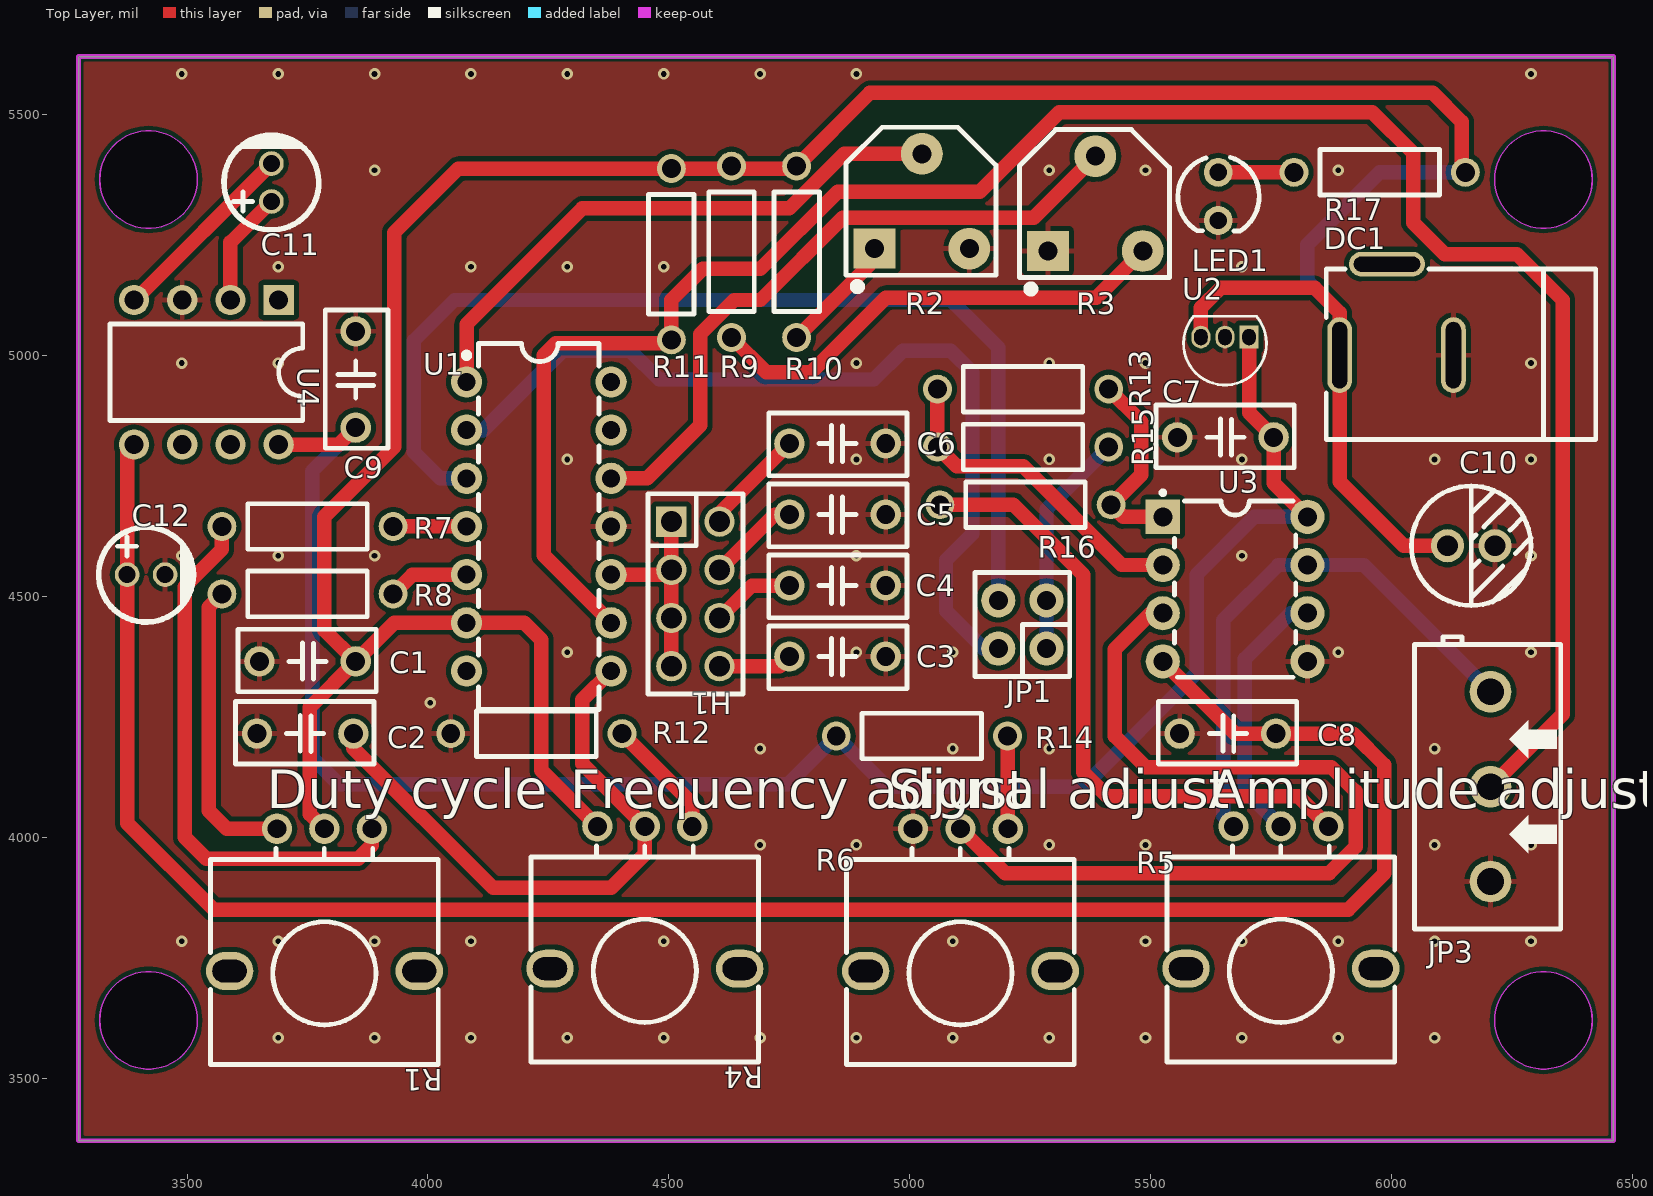
[diagram p0: Top Layer view]
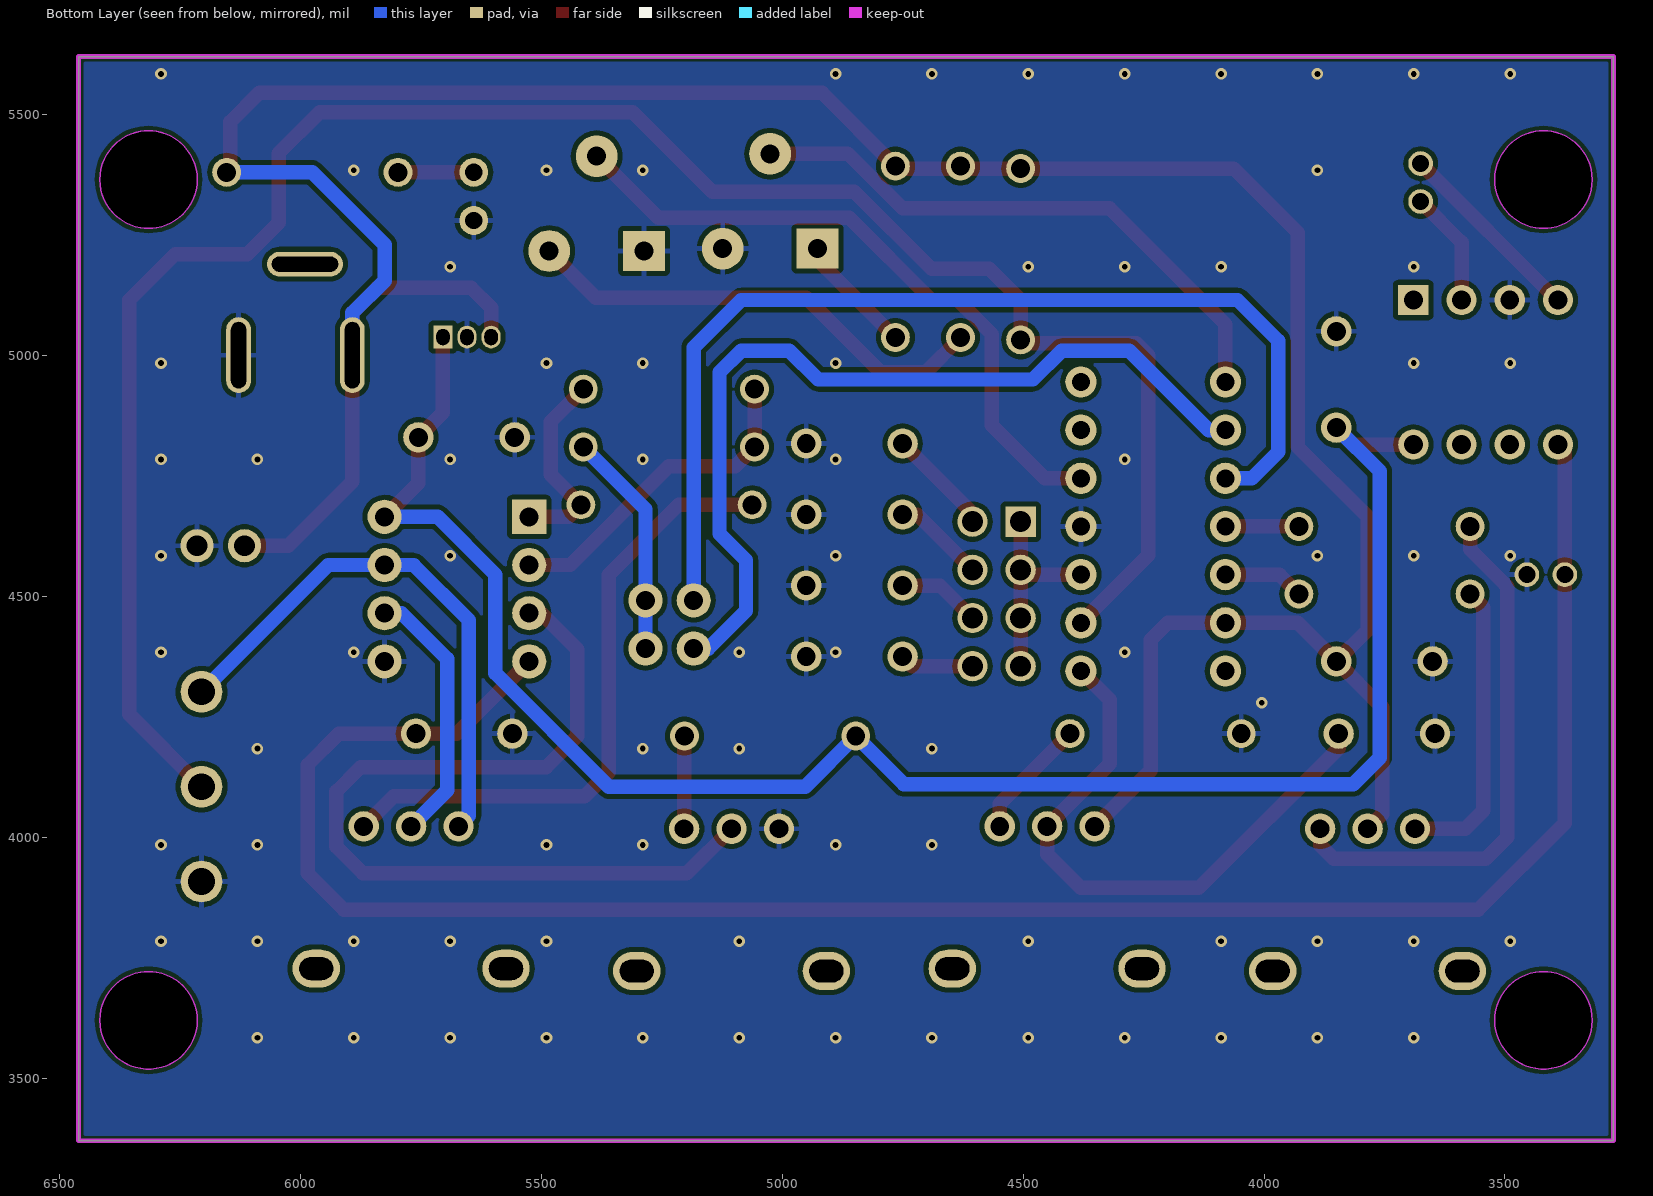
[diagram p1: Bottom Layer view, seen from below]
# Altium PCB MISC49930.pcbdoc
Units mil, origin at the board's own origin, x right, y up, seen from the top; angles counter-clockwise.
Board outline 3185 x 2250 mil, 2 copper layers (Top Layer, Bottom Layer), stack 62.206 mil thick; 38 components, 33 nets, 125 pads, 76 vias.

## Layer stack, top to bottom
Top Solder Mask Layer: solder mask 0.394, Dk 3.3
Top Layer: signal copper 1.379
Dielectric1: surface 59.449, FR4, Dk 4.5
Bottom Layer: signal copper 1.378
Bottom Solder Mask Layer: solder mask 0.394, Dk 3.3

## Board outline
3275,5620 3275,3370 6460,3370 6460,5620
cut-out: 3521.24,3620 cw(c3420,3620) 3318.76,3620 cw(c3420,3620)
cut-out: 3521.24,5365 cw(c3420,5365) 3318.76,5365 cw(c3420,5365)
cut-out: 6416.24,5365 cw(c6315,5365) 6213.76,5365 cw(c6315,5365)
cut-out: 6416.24,3620 cw(c6315,3620) 6213.76,3620 cw(c6315,3620)

## Design rules (kind name [scope] priority, off if disabled: settings)
BoardOutlineClearance copperThickness2oz_1 [All] p2 off: genericclearance=7.99 ignorepadtopadclearanceinfootprint=FALSE except(0: Arc-SplitContinuation Track-SplitContinuation SMDPad-SplitContinuation THPad-SplitContinuation Via-SplitContinuation Fill-SplitContinuation Region-SplitContinuation Poly-SplitContinuation Text-SplitContinuation Hole-SplitContinuation; 5.98: Arc-CutoutEdge SMDPad-CutoutEdge THPad-CutoutEdge Via-CutoutEdge Fill-CutoutEdge Region-CutoutEdge Text-CutoutEdge; 6.93: Hole-OutlineEdge Hole-CutoutEdge; 10: Poly-OutlineEdge Poly-CutoutEdge; 11.81: Arc-OutlineEdge Track-OutlineEdge SMDPad-OutlineEdge THPad-OutlineEdge Via-OutlineEdge Fill-OutlineEdge Region-OutlineEdge Text-OutlineEdge Track-CutoutEdge)
BoardOutlineClearance copperThickness1oz_1 [All] p4: genericclearance=4.02 ignorepadtopadclearanceinfootprint=FALSE except(0: Arc-SplitContinuation Track-SplitContinuation SMDPad-SplitContinuation THPad-SplitContinuation Via-SplitContinuation Fill-SplitContinuation Region-SplitContinuation Poly-SplitContinuation Text-SplitContinuation Hole-SplitContinuation; 6: SMDPad-CutoutEdge THPad-CutoutEdge Via-CutoutEdge Fill-CutoutEdge Region-CutoutEdge Text-CutoutEdge; 6.93: Hole-OutlineEdge Hole-CutoutEdge; 10: Poly-OutlineEdge Poly-CutoutEdge; 11.8: Arc-OutlineEdge Track-OutlineEdge SMDPad-OutlineEdge THPad-OutlineEdge Via-OutlineEdge Fill-OutlineEdge Region-OutlineEdge Text-OutlineEdge; 11.81: Arc-CutoutEdge Track-CutoutEdge)
Clearance copperThickness2oz [All] p1 off: gap=7.99 ignorepadtopadclearanceinfootprint=FALSE except(5.98: SMDPad-Track SMDPad-SMDPad THPad-Track SMDPad-THPad THPad-THPad Track-Via SMDPad-Via THPad-Via Via-Via Fill-Track Region-Track Fill-SMDPad Region-SMDPad Fill-THPad Region-THPad Fill-Via Region-Via Fill-Fill Fill-Region Region-Region Arc-Track Arc-SMDPad Arc-THPad Arc-Via Fill-Arc Region-Arc Arc-Arc Text-Track SMDPad-Text Text-THPad Text-Via Fill-Text Region-Text Arc-Text Text-Text; 6.93: Hole-Track Hole-SMDPad Hole-THPad Hole-Via Fill-Hole Region-Hole Hole-Arc Hole-Text; 10: Poly-Track Poly-SMDPad Poly-THPad Poly-Via Poly-Fill Poly-Region Poly-Poly Poly-Arc Poly-Text Poly-Hole)
Clearance copperThickness1oz [All] p3: gap=4.02 ignorepadtopadclearanceinfootprint=FALSE except(5.98: SMDPad-Track SMDPad-SMDPad THPad-Track SMDPad-THPad THPad-THPad Track-Via SMDPad-Via THPad-Via Via-Via Fill-Track Region-Track Fill-SMDPad Region-SMDPad Fill-THPad Region-THPad Fill-Via Region-Via Fill-Fill Fill-Region Region-Region; 6: Arc-Track Arc-SMDPad Arc-THPad Arc-Via Fill-Arc Region-Arc Arc-Arc Text-Track SMDPad-Text Text-THPad Text-Via Fill-Text Region-Text Arc-Text Text-Text; 6.93: Hole-Track Hole-SMDPad Hole-THPad Hole-Via Fill-Hole Region-Hole Hole-Arc Hole-Text; 10: Poly-Track Poly-SMDPad Poly-THPad Poly-Via Poly-Fill Poly-Region Poly-Poly Poly-Arc Poly-Text Poly-Hole)
Creepage creepage [All] p1: checkdistance=0 ignoreinternallayers=TRUE applytopolygonpour=TRUE
DiffPairsRouting differentialPair [All] p1: maxlimit=6 minlimit=6 mostfreqgap=6 toplayer_minwidth=5 toplayer_prefwidth=10 toplayer_maxwidth=100 toplayer_mingap=6 toplayer_prefgap=6 toplayer_maxgap=6 bottomlayer_minwidth=5 bottomlayer_prefwidth=10 bottomlayer_maxwidth=100 bottomlayer_mingap=6 bottomlayer_prefgap=6 bottomlayer_maxgap=6 maxuncoupledlength=10
HoleToHoleClearance otherClearance [All] p1: gap=11.81 allowstackedmicrovias=TRUE
Length netLength [All] p1: minlimit=0 maxlimit=0
MatchedLengths netLengthTolerance [All] p1: tolerance=1000
PasteMaskExpansion pasteMaskExpansion [All] p1: expansion=0
PlaneConnect innerPlane [All] p1: planeconnectstyle=Relief reliefexpansion=20 reliefentries=4 reliefconductorwidth=10 reliefairgap=10
PolygonConnect copperRegion [All] p1: connectstyle=Relief reliefconductorwidth=10 reliefentries=4 polygonreliefangle="90 Angle" airgapwidth=10 via.connectstyle=Relief via.reliefconductorwidth=10 via.reliefentries=4 via.polygonreliefangle="90 Angle" via.airgapwidth=10
RoutingVias viaSize [All] p1: holewidth=12.01 width=24.02 viastyle="Through Hole" minholewidth=11.81 minwidth=19.68 maxholewidth=248.03 maxwidth=393.7
SolderMaskExpansion solderMaskExpansion [IsVia] p1: expansion=-1000 istentingtop=TRUE
SolderMaskExpansion solderMaskExpansion [All] p2: expansion=2 istentingtop=FALSE
Width copperThickness2oz_2 [All] p1 off: maxlimit=100 minlimit=8 preferedwidth=10
Width copperThickness1oz_2 [All] p2: maxlimit=100 minlimit=5 preferedwidth=10

## Components (designator, comment, footprint, x,y, rotation, side; value= is the part's Value field where it differs from the comment)
C1 "100nF" CAP-TH_L5.1-W3.2-P5.08-D0.50 3750,4365 r0 top
C2 "100nF" CAP-TH_L5.1-W3.2-P5.08-D0.50 3745,4215 r0 top
C3 "101" CAP-TH_L5.1-W3.2-P5.08-D0.50 4850,4375 r180 top
C4 "101" CAP-TH_L5.1-W3.2-P5.08-D0.50 4850,4522.37 r180 top
C5 "101" CAP-TH_L5.1-W3.2-P5.08-D0.50 4850,4669.75 r180 top
C6 "101" CAP-TH_L5.1-W3.2-P5.08-D0.50 4850,4817.12 r180 top
C7 "100nF" CAP-TH_L5.1-W3.2-P5.08-D0.50 5655,4830 r0 top
C8 "100nF" CAP-TH_L5.1-W3.2-P5.08-D0.50 5660,4215 r0 top
C9 "100nF" CAP-TH_L5.1-W3.2-P5.08-D0.50 3850,4950 r270 top
C10 "100uF" CAP-TH_BD6.3-P2.5-D0.6-FD-RYHG35V100UF 6165,4605 r0 top
C11 "10uF" CAP-TH_BD5.0-P2.00-D0.8-FD-10UF50VC110GL 3675,5358.74 r90 top
C12 "10uF" CAP-TH_BD5.0-P2.00-D0.8-FD-10UF50VC110GL 3415,4545 r0 top
DC1 "" DC-2.0 6015,4990 r0 top
H1 "" HDR-TH_8P-P2.54-V-F-R2-C4-S2.54-1 4555,4505 r270 top
JP1 "" HDR-TH_4P-P2.54-V-F-R2-C2-S2.54 5233.6,4441.59 r90 top
JP3 "" CONN-TH_3P-P5.00_KF301-5.0-3P 6205,4105 r90 top
LED1 "" LED_TH-3mm 5640,5330 r270 top
R1 "10kΩ" RES-ADJ-TH_R09512N0-FB15A7.0-B103-005 3785,3870 r180 top
R2 "100kΩ" RES-ADJ-SMD_RM065-V1 5025,5320 r0 top
R3 "100kΩ" RES-ADJ-SMD_RM065-V1 5385,5315 r0 top
R4 "10kΩ" RES-ADJ-TH_R09512N0-FB15A7.0-B103-005 4450,3875 r180 top
R5 "10kΩ" RES-ADJ-TH_R09512N0-FB15A7.0-B103-005 5770,3875 r180 top
R6 "10kΩ" RES-ADJ-TH_R09512N0-FB15A7.0-B103-005 5105,3870 r180 top
R7 "1kΩ" Res_1/4W 3750,4645 r0 top
R8 "10kΩ" Res_1/4W 3750,4505 r0 top
R9 "10kΩ" Res_1/4W 4630,5215 r270 top
R10 "10kΩ" Res_1/4W 4765,5215 r90 top
R11 "4.7kΩ" Res_1/4W 4505,5210 r90 top
R12 "30kΩ" Res_1/4W 4225,4215 r0 top
R13 "10kΩ" Res_1/4W 5235,4930 r180 top
R14 "4.7kΩ" Res_1/4W 5025,4210 r0 top
R15 "10kΩ" Res_1/4W 5235,4810 r0 top
R16 "10kΩ" Res_1/4W 5240,4690 r0 top
R17 "10kΩ" Res_1/4W 5975,5380 r0 top
U1 "ICL8038CCPD" PDIP-14_L19.2-W6.6-P2.54-LS7.6-BL 4230,4645 r270 top
U2 "78l09" TO-92-3_L4.5-W3.5-P1.27-L 5654.02,5038.05 r180 top
U3 "" DIP-8_L9.3-W6.4-P2.54-LS7.6-TL 5675,4515 r0 top
U4 "TC7660S" DIP-8_L10.0-W6.5-P2.54-LS7.6-BL 3540,4965 r180 top

## Footprints (in the part's own frame and the unit in brackets; to place one, negate y for a bottom-side part, rotate by r counter-clockwise, add the part's x,y. Pads: shape width x height; smd on the part's side, far side on the other; paste and mask are expansions set on the pad)
CAP-TH_BD5.0-P2.00-D0.8-FD-10UF50VC110GL [mm]
  round 1.3 hole 0.9 paste+0 mask+0.051: 1(-1,0) 2(1,0)
  silkscreen extent -2.5,-2.5 2.5,2.5
CAP-TH_BD6.3-P2.5-D0.6-FD-RYHG35V100UF [mm]
  round 1.75 hole 1.1 paste+0 mask+0.05: 1(-1.25,0) 2(1.25,0)
  silkscreen extent -3.15,-3.16 3.15,3.15
CAP-TH_L5.1-W3.2-P5.08-D0.50 [mm]
  round 1.6 hole 1 paste+0 mask+0.05: 1(-2.54,0) 2(2.54,0)
  silkscreen extent -3.67,-1.6 3.63,1.7
CONN-TH_3P-P5.00_KF301-5.0-3P [mm]
  round 2.2 hole 1.4: 1(-5,0) 2(0,0) 3(5,0)
  silkscreen extent -7.5,-3.7 7.9,4
DC-2.0 [mil]
  oval 157.5x51.2 hole 31.5 slot 137.8 at 0 deg paste+0 mask+2: 2(-24.7,199.5)
  oval 51.2x157.5 hole 31.5 slot 137.8 at 90 deg paste+0 mask+2: 3(113.1,10.5) 4(-123.1,10.5)
  silkscreen extent -151,-165 408,190
DIP-8_L9.3-W6.4-P2.54-LS7.6-TL [mm]
  rect 1.8x1.8 hole 1: 1(-3.81,3.81)
  round 1.8 hole 1: 2(-3.81,1.27) 3(-3.81,-1.27) 4(-3.81,-3.81) 5(3.81,-3.81) 6(3.81,-1.27) 7(3.81,1.27) 8(3.81,3.81)
  silkscreen extent -3.91,-4.65 3.2,5.18
DIP-8_L10.0-W6.5-P2.54-LS7.6-BL [mil]
  rect 63x63 hole 39.37: 1(-150,-150)
  round 63 hole 39.37: 2(-50,-150) 3(50,-150) 4(150,-150) 5(150,150) 6(50,150) 7(-50,150) 8(-150,150)
  silkscreen extent -200,-100 200,100
HDR-TH_4P-P2.54-V-F-R2-C2-S2.54 [mm]
  round 1.8 hole 1: 1(-1.27,-1.27) 2(-1.27,1.27) 3(1.27,-1.27) 4(1.27,1.27)
  silkscreen extent -2.74,-2.5 2.74,2.5
HDR-TH_8P-P2.54-V-F-R2-C4-S2.54-1 [mm]
  rect 1.6x1.6 hole 1.1: 1(-3.81,-1.27)
  round 1.6 hole 1.1: 2(-3.81,1.27) 3(-1.27,-1.27) 4(-1.27,1.27) 5(1.27,-1.27) 6(1.27,1.27) 7(3.81,-1.27) 8(3.81,1.27)
  silkscreen extent -5.28,-2.5 5.28,2.5
LED_TH-3mm [mil]
  round 60 hole 36 paste+0 mask+2: 1(-50,0) 2(50,0)
  silkscreen extent -81,-84 72,85
PDIP-14_L19.2-W6.6-P2.54-LS7.6-BL [mm]
  round 1.65 hole 0.95: 1(-7.62,-3.81) 2(-5.08,-3.81) 3(-2.54,-3.81) 4(0,-3.81) 5(2.54,-3.81) 6(5.08,-3.81) 7(7.62,-3.81) 8(7.62,3.81) 9(5.08,3.81) 10(2.54,3.81) 11(0,3.81) 12(-2.54,3.81) 13(-5.08,3.81) 14(-7.62,3.81)
  silkscreen extent -9.65,-3.96 9.65,3.17
RES-ADJ-SMD_RM065-V1 [mm]
  rect 2.2x2.1 hole 1 paste+0 mask+0.05: 1(-2.5,-2.5)
  round 2.2 hole 1 paste+0 mask+0.05: 2(0,2.5) 3(2.5,-2.5)
  silkscreen extent -4,-4.7 3.9,3.9
RES-ADJ-TH_R09512N0-FB15A7.0-B103-005 [mm]
  round 1.6 hole 1: 1(-2.5,-3.75) 2(0,-3.75) 3(2.5,-3.75)
  oval 2.5x2 hole 1.2 slot 1.8 at 0 deg: 4(-5,3.75) 5(5,3.75)
  silkscreen extent -6,-2.72 6,8.67
Res_1/4W [mil]
  round 60 hole 39.37 paste+0 mask+2: 1(-177.76,0) 2(177.76,0)
  silkscreen extent -124,-47 124,47
TO-92-3_L4.5-W3.5-P1.27-L [mm]
  rect 1x1.2 hole 0.7 slot 0.85 at 90 deg: 1(-1.27,0)
  oval 1x1.2 hole 0.7 slot 0.85 at 90 deg: 2(0,0) 3(1.27,0)
  silkscreen extent -2.19,-1.1 2.19,2.52

## Via types
v1: diameter 24.02, hole 12, Top Layer to Bottom Layer, 76 vias

## Nets (pads, with @x,y where several pads share a name; then routed paths per layer and width w, separated by ;. In a path a pad name is that pad's centre, name@x,y a point inside that pad or via, vN(x,y) a via of type N, cw(c..) or ccw(c..) an arc to the next point about the centre after c; other vN are vias at no path point)
$1N4: LED1.1 R17.1 | length 157.2
  Top Layer w30: LED1.1 R17.1
$1N14: C11.2 U4.4 | length 402.3
  Top Layer w30: U4.4 3391.89,5115 C11.2
$1N15: C11.1 U4.2 | length 239.6
  Top Layer w30: U4.2 3590,5234.37 C11.1
$1N18: R7.2 U1.4 | length 152.2
  Top Layer w30: R7.2 U1.4
$1N19: R1.1 R7.1 | length 1130
  Top Layer w30: R7.1 3572.24,4597.24 3500.94,4525.94 3500.94,4525.71 3495,4519.76 3495,4000 3540,3955 3855,3955 3883.42,3983.42 R1.1
$1N21: R1.3 R8.1 | length 618.3
  Top Layer w30: R8.1 3545,4477.76 3545,4055 3582.36,4017.64 R1.3
$1N22: R8.2 U1.5 | length 168.8
  Top Layer w30: R8.2 3967.76,4545 U1.5
$1N24: R6.1 R14.2 | length 192.6
  Top Layer w30: R14.2 5202.76,4018.3 R6.1
$1N25: R6.2 U3.3 | length 1854.9
  Top Layer w30: R6.2 5197.64,3925 5870,3925 5925,3980 5925,4095 5875,4145 5490,4145 5425,4210 5425,4390 5500,4465 U3.3
$1N27: C6.2 H1.2 | length 222.2
  Top Layer w30: H1.2 4605,4672.12 C6.2
$1N28: C5.2 H1.4 | length 192.5
  Top Layer w30: H1.4 4719.75,4669.75 C5.2
$1N29: C3.2 H1.8 | length 153.3
  Top Layer w30: H1.8 4730,4355 C3.2
$1N30: C4.2 H1.6 | length 172.9
  Top Layer w30: H1.6 4672.37,4522.37 C4.2
$1N32: R4.1 R12.2 | length 252.7
  Top Layer w30: R12.2 4548.42,4069.34 R4.1
$1N34: C2.2 R4.2 U1.8 | length 1242.8
  Top Layer w30: C2.2 3845,4185 4135,3895 4380,3895 4450,3965 R4.2 4320,4152.64 4320,4285 U1.8
$1N36: H1.1 H1.3 H1.5 H1.7 U1.10 | length 429.1
  Top Layer w30: U1.10 4495,4545 H1.3 ; H1.7 H1.5 H1.3 ; H1.1 H1.3
$1N38: R3.2 U1.12 | length 1392.8
  Top Layer w30: U1.12 4455,4745 4565,4855 4565,5044.34 4635.66,5115 4690,5115 4860.87,5285.87 5257.44,5285.87 R3.2
$1N39: R3.3 R9.2 | length 987.6
  Top Layer w30: R9.2 4702.24,4965 4795,4965 4950,5120 5386.85,5120 R3.3
$1N41: R2.1 R10.1 | length 251.3
  Top Layer w30: R10.1 4926.57,5198.81 R2.1
$1N42: R2.2 U1.1 | length 1211.4
  Top Layer w30: U1.1 4080,5065 4320,5305 4750,5305 4863.43,5418.43 R2.2
$1N43: JP1.2 U1.2 | length 1845.6
  Bottom Layer w30: U1.2 4115,4845 4280,5010 4420,5010 4480,4950 4925,4950 4985,5010 5085,5010 5130,4965 5130,4630 5075,4575 5075,4470 5153.41,4391.59 JP1.2
$1N44: JP1.4 U1.3 | length 2177.2
  Bottom Layer w30: U1.3 4025,4745 3970,4800 3970,5030 4055,5115 5085,5115 5183.6,5016.4 JP1.4
$1N45: JP1.1 JP1.3 R15.2 | length 471.9
  Bottom Layer w30: JP1.1 JP1.3 5283.6,4680.84 R15.2
$1N46: R13.2 R15.1 U3.2 | length 689.2
  Top Layer w30: R13.2 R15.1 5097.24,4770 5235,4770 5440,4565 U3.2
$1N49: R13.1 R16.2 U3.1 | length 411.2
  Top Layer w30: R13.1 5480,4862.76 5480,4752.24 R16.2 5442.76,4665 U3.1
$1N50: R5.1 R16.1 | length 1322.8
  Top Layer w30: R16.1 5215,4690 5360,4545 5360,4135 5410,4085 5806.06,4085 R5.1
$1N51: R5.2 U3.6 | length 547.8
  Bottom Layer w30: R5.2 5695,4097.64 5695,4370 5790,4465 U3.6
$1N52: JP3.3 R5.3 U3.7 | length 1147.9
  Bottom Layer w30: R5.3 5650,4044.2 5650,4450 5765,4565 U3.7 5941.85,4565 JP3.3
+9V: C7.2 C9.2 R14.1 U2.1 U3.8 U4.8 | length 3844.7
  Top Layer w30: U4.8 3815,4815 C9.2 ; U2.1 5704.02,4880.98 C7.2 5755,4735 U3.8
  Bottom Layer w30: C9.2 3760,4760 3760,4165 3815,4110 4747.24,4110 R14.1 4952.24,4105 5360,4105 5595,4340 5595,4545 5715,4665 U3.8
+12V: C1.2 C10.1 DC1.4 R1.2 R4.3 R9.1 R10.2 R11.2 R17.2 U1.6 U2.3 | length 6376.1
  Top Layer w30: R1.2 3755,4047.64 3755,4270 C1.2 ; R4.3 4235,4139.2 4235,4410 4200,4445 U1.6 3930,4445 C1.2 ; U2.3 5604.02,5099.02 5645,5140 5840,5140 5891.9,5088.1 DC1.4 5891.9,4738.1 6025,4605 C10.1 ; R17.2 6145,5387.76 6145,5485 6085,5545 4917.24,5545 R10.2 4760,5387.76 R11.2 4062.76,5387.76 3930,5255 3930,4810 3785,4665 3785,4430 C1.2
  Bottom Layer w30: DC1.4 5891.9,5088.1 5825,5155 5825,5230 5975,5380 R17.2
-9V: C8.2 C12.1 U3.4 U4.5 | length 4280.4
  Top Layer w30: U4.5 3375.63,4800.63 C12.1 3375.63,4029.37 3555,3850 5910,3850 5985,3925 5985,4150 5920,4215 C8.2 5675,4215 U3.4
GND: C1.1 C2.1 C3.1 C4.1 C5.1 C6.1 C7.1 C8.1 C9.1 C10.2 C12.2 DC1.3 JP3.1 LED1.2 R2.3 R3.1 R6.3 R12.1 U1.11 U2.2 U3.5 U4.3
  other v1: 3689.1,3584.1 3889.1,3584.1 4089.1,3584.1 4289.1,3584.1 4489.1,3584.1 4689.1,3584.1 4889.1,3584.1 5089.1,3584.1 5289.1,3584.1 5489.1,3584.1 5689.1,3584.1 5889.1,3584.1 6089.1,3584.1 3489.1,3784.1 3689.1,3784.1 3889.1,3784.1 4089.1,3784.1 4489.1,3784.1 5089.1,3784.1 5489.1,3784.1 5689.1,3784.1 5889.1,3784.1 6089.1,3784.1 6289.1,3784.1 4689.1,3984.1 4889.1,3984.1 5289.1,3984.1 5489.1,3984.1 6089.1,3984.1 6289.1,3984.1 4689.1,4184.1 5089.1,4184.1 5289.1,4184.1 6089.1,4184.1 4004.73,4279.1 4289.1,4384.1 4889.1,4384.1 5089.1,4384.1 5889.1,4384.1 6289.1,4384.1 3489.1,4584.1 3689.1,4584.1 3889.1,4584.1 4889.1,4584.1 5689.1,4584.1 6289.1,4584.1 4289.1,4784.1 4889.1,4784.1 5289.1,4784.1 5689.1,4784.1 6089.1,4784.1 6289.1,4784.1 3489.1,4984.1 3689.1,4984.1 4889.1,4984.1 5289.1,4984.1 5489.1,4984.1 6289.1,4984.1 3689.1,5184.1 4089.1,5184.1 4289.1,5184.1 4489.1,5184.1 5689.1,5184.1 3889.1,5384.1 5289.1,5384.1 5489.1,5384.1 5889.1,5384.1 3489.1,5584.1 3689.1,5584.1 3889.1,5584.1 4089.1,5584.1 4289.1,5584.1 4489.1,5584.1 4689.1,5584.1 4889.1,5584.1 6289.1,5584.1
SQUOUT: JP3.2 R11.1 U1.9 | length 4304.3
  Top Layer w30: U1.9 4240,4585.01 4240,5000 4265,5025 4497.76,5025 R11.1 4505,5115 4570,5180 4690,5180 4850,5340 5145,5340 5310,5505 5960,5505 6045,5420 6045,5275 6110,5210 6260,5210 6355,5115 6355,4255 JP3.2
pads on no net: DC1.2 R1.4 R1.5 R4.4 R4.5 R5.4 R5.5 R6.4 R6.5 U1.7 U1.13 U1.14 U4.1 U4.6 U4.7

## Polygon pours and split planes (outlines as drawn)
GND on Top Layer (solid, remove dead copper, pour order 2): 3000,5850 3000,3100 6735,3100 6735,5850
GND on Bottom Layer (solid, remove dead copper, pour order 4): 3045,5855 3045,3000 6850,3000 6850,5855

## Keep-outs
Board Outline Layer:
  region: 3521.24,3620 cw(c3420,3620) 3318.76,3620 cw(c3420,3620)
  circle w0.1: c3420,3620 r101.24
  region: 3521.24,3620 3520.86,3611.18 3519.7,3602.42 3517.79,3593.8 3515.14,3585.37 3511.76,3577.21 3507.68,3569.38 3502.93,3561.93 3497.56,3554.92 3491.59,3548.41 3485.08,3542.44 3478.07,3537.07 3470.62,3532.32 3462.79,3528.24 3454.63,3524.86 3446.2,3522.21 3437.58,3520.3 3428.82,3519.14 3420,3518.76 3411.18,3519.14 3402.42,3520.3 3393.8,3522.21 3385.37,3524.86 3377.21,3528.24 3369.38,3532.32 3361.93,3537.07 3354.92,3542.44 3348.41,3548.41 3342.44,3554.92 3337.07,3561.93 3332.32,3569.38 3328.24,3577.21 3324.86,3585.37 3322.21,3593.8 3320.3,3602.42 3319.14,3611.18 3318.76,3620 3319.14,3628.82 3320.3,3637.58 3322.21,3646.2 3324.86,3654.63 3328.24,3662.79 3332.32,3670.62 3337.07,3678.07 3342.44,3685.08 3348.41,3691.59 3354.92,3697.56 3361.93,3702.93 3369.38,3707.68 3377.21,3711.76 3385.37,3715.14 3393.8,3717.79 3402.42,3719.7 3411.18,3720.86 3420,3721.24 3428.82,3720.86 3437.58,3719.7 3446.2,3717.79 3454.63,3715.14 3462.79,3711.76 3470.62,3707.68 3478.07,3702.93 3485.08,3697.56 3491.59,3691.59 3497.56,3685.08 3502.93,3678.07 3507.68,3670.62 3511.76,3662.79 3515.14,3654.63 3517.79,3646.2 3519.7,3637.58 3520.86,3628.82
  region: 3521.24,5365 cw(c3420,5365) 3318.76,5365 cw(c3420,5365)
  circle w0.1: c3420,5365 r101.24
  region: 3521.24,5365 3520.86,5356.18 3519.7,5347.42 3517.79,5338.8 3515.14,5330.37 3511.76,5322.21 3507.68,5314.38 3502.93,5306.93 3497.56,5299.92 3491.59,5293.41 3485.08,5287.44 3478.07,5282.07 3470.62,5277.32 3462.79,5273.24 3454.63,5269.86 3446.2,5267.21 3437.58,5265.3 3428.82,5264.14 3420,5263.76 3411.18,5264.14 3402.42,5265.3 3393.8,5267.21 3385.37,5269.86 3377.21,5273.24 3369.38,5277.32 3361.93,5282.07 3354.92,5287.44 3348.41,5293.41 3342.44,5299.92 3337.07,5306.93 3332.32,5314.38 3328.24,5322.21 3324.86,5330.37 3322.21,5338.8 3320.3,5347.42 3319.14,5356.18 3318.76,5365 3319.14,5373.82 3320.3,5382.58 3322.21,5391.2 3324.86,5399.63 3328.24,5407.79 3332.32,5415.62 3337.07,5423.07 3342.44,5430.08 3348.41,5436.59 3354.92,5442.56 3361.93,5447.93 3369.38,5452.68 3377.21,5456.76 3385.37,5460.14 3393.8,5462.79 3402.42,5464.7 3411.18,5465.86 3420,5466.24 3428.82,5465.86 3437.58,5464.7 3446.2,5462.79 3454.63,5460.14 3462.79,5456.76 3470.62,5452.68 3478.07,5447.93 3485.08,5442.56 3491.59,5436.59 3497.56,5430.08 3502.93,5423.07 3507.68,5415.62 3511.76,5407.79 3515.14,5399.63 3517.79,5391.2 3519.7,5382.58 3520.86,5373.82
  region: 6416.24,5365 cw(c6315,5365) 6213.76,5365 cw(c6315,5365)
  circle w0.1: c6315,5365 r101.24
  region: 6416.24,5365 6415.86,5356.18 6414.7,5347.42 6412.79,5338.8 6410.14,5330.37 6406.76,5322.21 6402.68,5314.38 6397.93,5306.93 6392.56,5299.92 6386.59,5293.41 6380.08,5287.44 6373.07,5282.07 6365.62,5277.32 6357.79,5273.24 6349.63,5269.86 6341.2,5267.21 6332.58,5265.3 6323.82,5264.14 6315,5263.76 6306.18,5264.14 6297.42,5265.3 6288.8,5267.21 6280.37,5269.86 6272.21,5273.24 6264.38,5277.32 6256.93,5282.07 6249.92,5287.44 6243.41,5293.41 6237.44,5299.92 6232.07,5306.93 6227.32,5314.38 6223.24,5322.21 6219.86,5330.37 6217.21,5338.8 6215.3,5347.42 6214.14,5356.18 6213.76,5365 6214.14,5373.82 6215.3,5382.58 6217.21,5391.2 6219.86,5399.63 6223.24,5407.79 6227.32,5415.62 6232.07,5423.07 6237.44,5430.08 6243.41,5436.59 6249.92,5442.56 6256.93,5447.93 6264.38,5452.68 6272.21,5456.76 6280.37,5460.14 6288.8,5462.79 6297.42,5464.7 6306.18,5465.86 6315,5466.24 6323.82,5465.86 6332.58,5464.7 6341.2,5462.79 6349.63,5460.14 6357.79,5456.76 6365.62,5452.68 6373.07,5447.93 6380.08,5442.56 6386.59,5436.59 6392.56,5430.08 6397.93,5423.07 6402.68,5415.62 6406.76,5407.79 6410.14,5399.63 6412.79,5391.2 6414.7,5382.58 6415.86,5373.82
  region: 6416.24,3620 cw(c6315,3620) 6213.76,3620 cw(c6315,3620)
  circle w0.1: c6315,3620 r101.24
  region: 6416.24,3620 6415.86,3611.18 6414.7,3602.42 6412.79,3593.8 6410.14,3585.37 6406.76,3577.21 6402.68,3569.38 6397.93,3561.93 6392.56,3554.92 6386.59,3548.41 6380.08,3542.44 6373.07,3537.07 6365.62,3532.32 6357.79,3528.24 6349.63,3524.86 6341.2,3522.21 6332.58,3520.3 6323.82,3519.14 6315,3518.76 6306.18,3519.14 6297.42,3520.3 6288.8,3522.21 6280.37,3524.86 6272.21,3528.24 6264.38,3532.32 6256.93,3537.07 6249.92,3542.44 6243.41,3548.41 6237.44,3554.92 6232.07,3561.93 6227.32,3569.38 6223.24,3577.21 6219.86,3585.37 6217.21,3593.8 6215.3,3602.42 6214.14,3611.18 6213.76,3620 6214.14,3628.82 6215.3,3637.58 6217.21,3646.2 6219.86,3654.63 6223.24,3662.79 6227.32,3670.62 6232.07,3678.07 6237.44,3685.08 6243.41,3691.59 6249.92,3697.56 6256.93,3702.93 6264.38,3707.68 6272.21,3711.76 6280.37,3715.14 6288.8,3717.79 6297.42,3719.7 6306.18,3720.86 6315,3721.24 6323.82,3720.86 6332.58,3719.7 6341.2,3717.79 6349.63,3715.14 6357.79,3711.76 6365.62,3707.68 6373.07,3702.93 6380.08,3697.56 6386.59,3691.59 6392.56,3685.08 6397.93,3678.07 6402.68,3670.62 6406.76,3662.79 6410.14,3654.63 6412.79,3646.2 6414.7,3637.58 6415.86,3628.82
  lines w10: 3275,3370 3275,5620 6460,5620 6460,3370 3275,3370

## Silkscreen, mask and mechanical layers (free items; w line width, h text height)
Top Silkscreen Layer:
  text "Duty cycle" at 3665,4060 h80
  text "Frequency adjust" at 4295,4060 h80
  text "Signal adjust" at 4955,4060 h80
  text "Amplitude adjust" at 5620,4060 h80
Mechanical Layer:
  circle w0.1: c3420,3620 r101.24
  circle w0.1: c3420,5365 r101.24
  circle w0.1: c6315,5365 r101.24
  circle w0.1: c6315,3620 r101.24